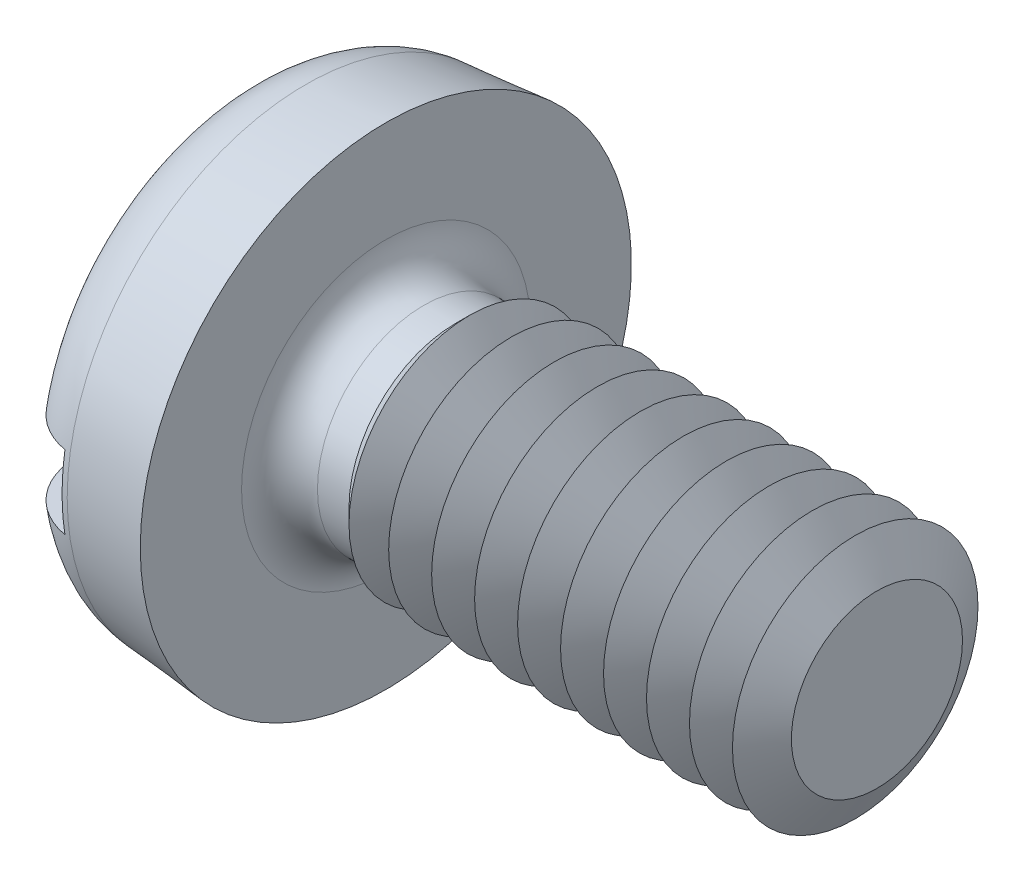
from build123d import *

# Parameters (mm, degrees)
SKETCH_4_W             = 1
SKETCH_4_H             = 1.2
CUT_EXTRUDE_1_DEPTH    = 50
PATTERN_LINEAR_1_COUNT = 10
PATTERN_LINEAR_1_PITCH = 0.7


with BuildPart() as part:
    # 草图3 → Revolve 915 (revolve)
    with BuildSketch(Plane.XY, mode=Mode.PRIVATE) as revolve_915_sk:
        with BuildLine():
            Line((0, 0), (10.4, 0))
            Line((10.4, 0), (10.4, 2))
            Line((10.4, 2), (3.8, 2))
            Line((3.8, 2), (3.532, 1.732))
            Line((3.532, 1.732), (3.018, 1.732))
            ThreePointArc((3.018, 1.732), (2.581008009, 1.913008009), (2.4, 2.35))
            Line((2.4, 2.35), (2.4, 4))
            Line((2.4, 4), (1.095413109, 3.885863436))
            ThreePointArc((1.095413109, 3.885863436), (0.315267196, 3.501138048), (0, 2.690429799))
            Line((0, 2.690429799), (0, 0))
        make_face()
    revolve(revolve_915_sk.sketch.rotate(Axis((-2.477021524, 0, 0), (1, 0, 0)), 90), axis=Axis((-2.477021524, 0, 0), (1, 0, 0)))

    # 草图4 → 切除-拉伸1 (cut, symmetric)
    with BuildSketch(Plane.XY):
        with Locations((0.5, 0)):
            Rectangle(SKETCH_4_W, SKETCH_4_H)
    extrude(amount=CUT_EXTRUDE_1_DEPTH, both=True, mode=Mode.SUBTRACT)

    # 草图5 → 切除-旋转1 (revolve, cut)
    with BuildSketch(Plane.XY, mode=Mode.PRIVATE) as cut_revolve_1_sk:
        Polygon((10.046208796, 2), (10.746208796, 2), (10.4, 1.3938), align=None)
    cut_revolve_1 = revolve(cut_revolve_1_sk.sketch.rotate(Axis((6.174994867, 0, 0), (-1, 0, 0)), 270), axis=Axis((6.174994867, 0, 0), (-1, 0, 0)), mode=Mode.SUBTRACT)

    # 阵列(线性)1: 切除-旋转1 ×10
    with Locations(*[(-i * PATTERN_LINEAR_1_PITCH, 0, 0) for i in range(1, PATTERN_LINEAR_1_COUNT)]):
        add(cut_revolve_1, mode=Mode.SUBTRACT)


solid = part.part
